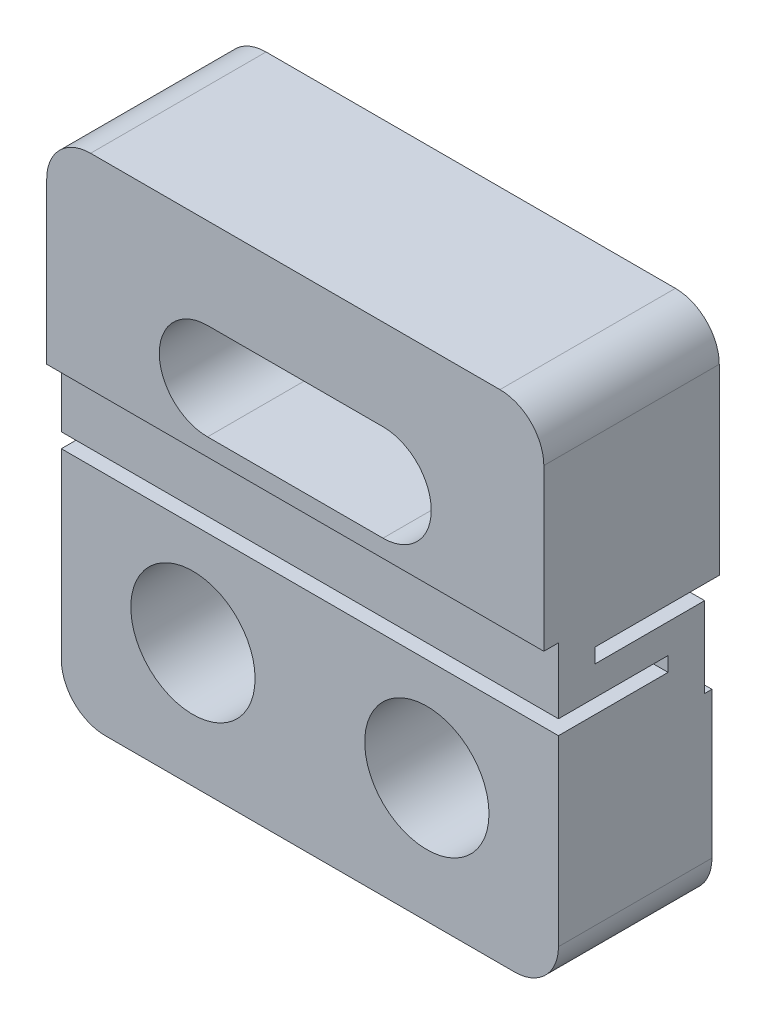
SolidWorks part; units mm, degrees
ref_plane "Front Plane" through (0, 0, 0) normal (0, 0, 1) x (1, 0, 0)
ref_plane "Top Plane" through (0, 0, 0) normal (0, 1, 0) x (1, 0, 0)
ref_plane "Right Plane" through (0, 0, 0) normal (1, 0, 0) x (0, 0, -1)
sketch "Sketch1" plane through (0, 0, 0) normal (0, 0, 1) x (1, 0, 0)
  line L1 (17, -17.5) -> (-17, -17.5)
  line L2 (17, -17.5) -> (17, 17.5)
  line L3 (17, 17.5) -> (-17, 17.5)
  line L4 (-17, -17.5) -> (-17, 17.5)
  line L5 (17, -17.5) -> (-17, 17.5) construction
  line L6 (17, 17.5) -> (-17, -17.5) construction
  point P0 (0, 0)
  dimension "D1" = 35
  dimension "D2" = 34
extrude "Boss-Extrude1" add sketch "Sketch1" along normal blind 12
sketch "Sketch2" plane through (0, 0, 12) normal (0, 0, 1) x (1, 0, 0)
  line L0 (0, 0) -> (0, 26.0725) construction
  line L1 (-6, 8) -> (6, 8) construction
  line L2 (-6, 11.3) -> (6, 11.3)
  line L3 (-6, 4.7) -> (6, 4.7)
  line L4 (17, 17.5) -> (-17, 17.5) construction
  line L5 (-17, -17.5) -> (17, -17.5) construction
  arc A0 (-6, 11.3) -> (-6, 4.7) centre (-6, 8) ccw
  arc A1 (6, 4.7) -> (6, 11.3) centre (6, 8) ccw
  circle A2 centre (-8, -9) radius 2.1
  circle A3 centre (8, -9) radius 2.1
  point P5 (0, 8)
  dimension "D4" = 4.2
  dimension "D6" = 4.2
  dimension "D1" = 9.5
  dimension "D2" = 12
  dimension "D3" = 6
  dimension "D5" = 8.5
  dimension "D7" = 16
  dimension "D8" = 8
extrude "Cut-Extrude1" cut sketch "Sketch2" against normal through all
sketch "Sketch3" plane through (0, 0, 12) normal (0, 0, 1) x (1, 0, 0)
  line L0 (-20.364, 3.5) -> (23.0197, 3.5)
  line L1 (23.0197, 3.5) -> (23.0197, -17.6868)
  line L2 (23.0197, -17.6868) -> (-20.364, -17.6868)
  line L3 (-20.364, -17.6868) -> (-20.364, 3.5)
  line L4 (17, 17.5) -> (-17, 17.5) construction
  dimension "D1" = 14
extrude "Cut-Extrude2" cut sketch "Sketch3" against normal blind 1
sketch "Sketch4" plane through (0, 0, 0) normal (0, 0, -1) x (-1, 0, 0)
  line L0 (-24.7629, -4.5) -> (25.8584, -4.5)
  line L1 (25.8584, -4.5) -> (25.8584, -22.3805)
  line L2 (25.8584, -22.3805) -> (-24.7629, -22.3805)
  line L3 (-24.7629, -22.3805) -> (-24.7629, -4.5)
  line L4 (17, -17.5) -> (-17, -17.5) construction
  dimension "D1" = 13
extrude "Cut-Extrude3" cut sketch "Sketch4" against normal blind 0.5
sketch "Sketch5" plane through (0, 0, 0) normal (0, 0, -1) x (-1, 0, 0)
  line L0 (-23.9126, 2) -> (26.338, 2)
  line L1 (17, -4.5) -> (-17, -4.5) construction
  line L2 (17, -4.5) -> (-17, -4.5)
  line L3 (-17, -4.5) -> (-23.9126, 2)
  line L4 (17, -4.5) -> (26.338, 2)
  dimension "D1" = 6.5
extrude "Cut-Extrude4" cut sketch "Sketch5" against normal blind 1
sketch "Sketch6" plane through (0, 0, 11) normal (0, 0, 1) x (1, 0, 0)
  circle A0 centre (8, -9) radius 4.25
  circle A1 centre (-8, -9) radius 4.25
  dimension "D1" = 8.5
  dimension "D2" = 8.5
extrude "Cut-Extrude5" cut sketch "Sketch6" against normal blind 6.5
sketch "Sketch7" plane through (0, 0, 1) normal (0, 0, -1) x (-1, 0, 0)
  line L0 (17, 2) -> (17, 1)
  line L1 (17, 2) -> (17, -4.5) construction
  line L2 (17, 1) -> (-18.6212, 1)
  line L3 (-18.6212, 1) -> (-18.6212, 2)
  line L4 (-18.6212, 2) -> (17, 2)
  dimension "D1" = 1
extrude "Cut-Extrude6" cut sketch "Sketch7" against normal offset from surface (7.5 mm away) 2.5 up to face at (12.25, -9, 11)
sketch "Sketch8" plane through (0, 0, 11) normal (0, 0, 1) x (1, 0, 0)
  line L0 (17, -2) -> (-17, -2)
  line L1 (17, 3.5) -> (17, -17.5) construction
  line L2 (-17, -17.5) -> (-17, 3.5) construction
  line L3 (-17, -2) -> (-17, -1)
  line L4 (-17, -1) -> (17, -1)
  line L5 (17, -1) -> (17, -2)
  line L6 (17, -17.5) -> (-17, -17.5) construction
  dimension "D1" = 1
  dimension "D2" = 15.5
extrude "Cut-Extrude7" cut sketch "Sketch8" against normal offset from surface (7.5 mm away) 2.5 up to face at (0, -1.75, 1)
fillet "Fillet1" radius 3 4 edges at (-17, -17.5, 5.75) (17, -17.5, 5.75) (17, 17.5, 6) (-17, 17.5, 6)
